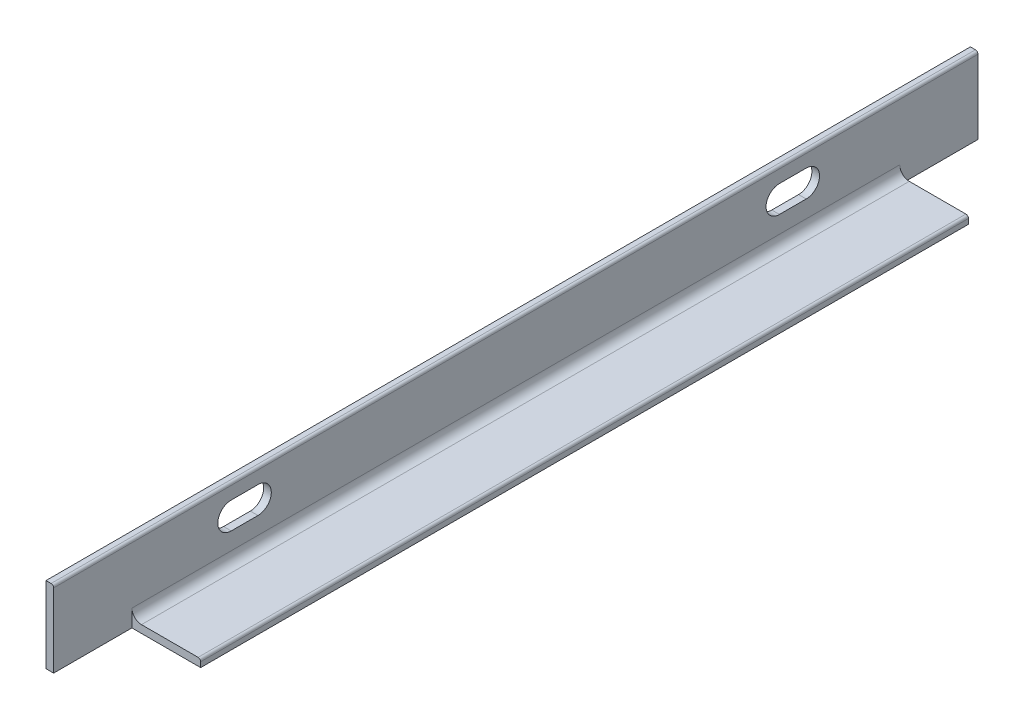
from build123d import *

# Parameters (mm, degrees)
EXTRUDE_THIN1_DEPTH = 484.14
FILLET1_R           = 5
FILLET2_R           = 1.333333333
SKETCH2_W           = 36
SKETCH2_H           = 41
CUT_EXTRUDE1_DEPTH  = 488.43362584
SKETCH3_W           = 36
SKETCH3_H           = 41
CUT_EXTRUDE3_DEPTH  = 488.43362584
CUT_EXTRUDE4_DEPTH  = 14
LPATTERN1_COUNT     = 2
LPATTERN1_PITCH     = 287.14


with BuildPart() as part:
    # Sketch1 → Extrude-Thin1 (new body)
    with BuildSketch(Plane.XY):
        Polygon((0, 40), (0, 0), (40, 0), (40, 4), (4, 4), (4, 40), align=None)
    extrude(amount=EXTRUDE_THIN1_DEPTH)

    # Fillet1
    fillet1_edges = [part.edges().sort_by_distance(p)[0] for p in [
        (4, 4, 242.07),
    ]]
    fillet(fillet1_edges, radius=FILLET1_R)

    # Fillet2
    fillet2_edges = [part.edges().sort_by_distance(p)[0] for p in [
        (40, 4, 242.07),
        (4, 40, 242.07),
    ]]
    fillet(fillet2_edges, radius=FILLET2_R)

    # Sketch2 → Cut-Extrude1 (cut, through all)
    with BuildSketch(Plane.XZ):
        with Locations((22, 20.5)):
            Rectangle(SKETCH2_W, SKETCH2_H)
    extrude(amount=-CUT_EXTRUDE1_DEPTH, mode=Mode.SUBTRACT)

    # Sketch3 → Cut-Extrude3 (cut, through all)
    with BuildSketch(Plane.XZ):
        with Locations((22, 463.64)):
            Rectangle(SKETCH3_W, SKETCH3_H)
    extrude(amount=-CUT_EXTRUDE3_DEPTH, mode=Mode.SUBTRACT)

    # Sketch4 → Cut-Extrude4 (cut)
    with BuildSketch(Plane(origin=(4, 0, 0), x_dir=(0, 0, -1), z_dir=(1, 0, 0))):
        with BuildLine():
            Line((-391.14, 32), (-377.14, 32))
            ThreePointArc((-377.14, 32), (-370.14, 25), (-377.14, 18))
            Line((-377.14, 18), (-391.14, 18))
            ThreePointArc((-391.14, 18), (-398.14, 25), (-391.14, 32))
        make_face()
    cut_extrude4 = extrude(amount=-CUT_EXTRUDE4_DEPTH, mode=Mode.SUBTRACT)

    # LPattern1: Cut-Extrude4 ×2
    with Locations(*[(0, 0, -i * LPATTERN1_PITCH) for i in range(1, LPATTERN1_COUNT)]):
        add(cut_extrude4, mode=Mode.SUBTRACT)


solid = part.part
